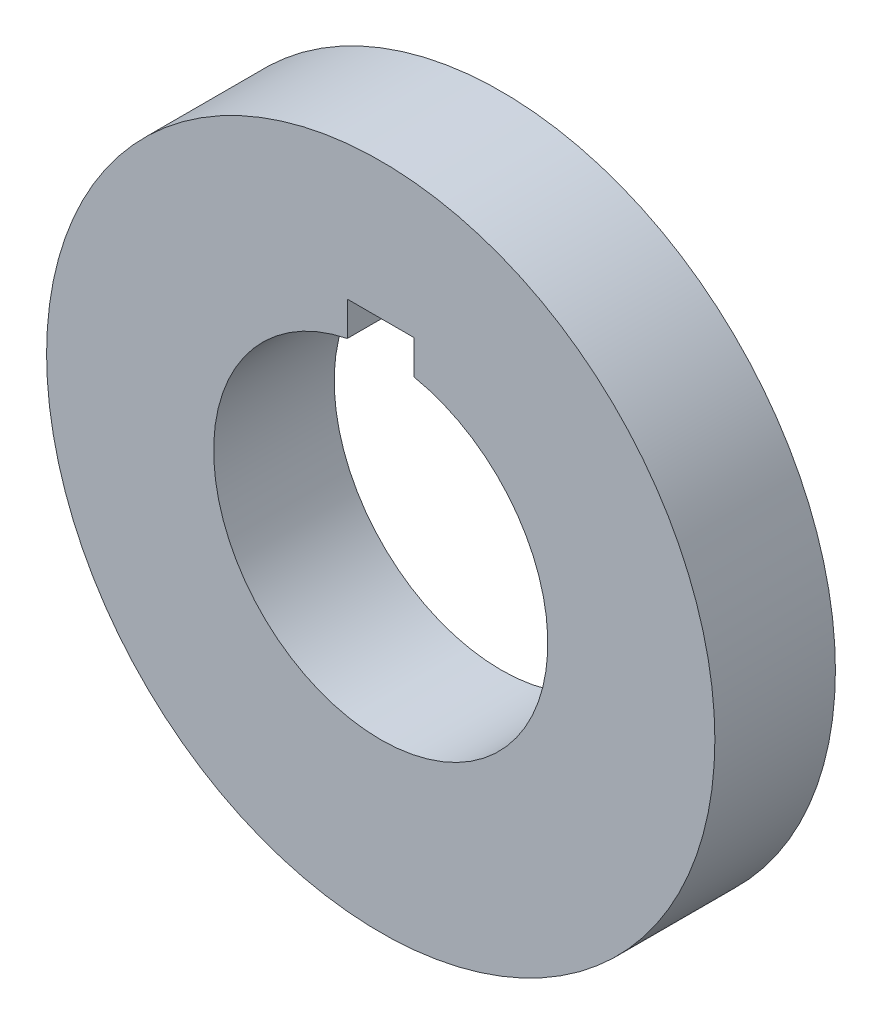
from build123d import *

# Parameters (mm, degrees)
SKETCH1_R           = 25
SKETCH1_R_2         = 12.5
BOSS_EXTRUDE1_DEPTH = 17
MOVE_FACE1_BY       = 7.981500203
SKETCH2_W           = 5
SKETCH2_H           = 4.6
CUT_EXTRUDE1_DEPTH  = 37.487440834


with BuildPart() as part:
    # Sketch1 → Boss-Extrude1 (new body)
    with BuildSketch(Plane.XY):
        Circle(SKETCH1_R)
        Circle(SKETCH1_R_2, mode=Mode.SUBTRACT)
    extrude(amount=-BOSS_EXTRUDE1_DEPTH)

    # Move Face1: a face moved inward by 7.9815
    extrude(part.faces().sort_by_distance((0, -20, 0))[0], amount=MOVE_FACE1_BY, dir=(0, 0, -1), mode=Mode.SUBTRACT)

    # Sketch2 → Cut-Extrude1 (cut, through all)
    with BuildSketch(Plane(origin=(0, 0, -17), x_dir=(-1, 0, 0), z_dir=(0, 0, -1))):
        with Locations((0, 12.5)):
            Rectangle(SKETCH2_W, SKETCH2_H)
    extrude(amount=-CUT_EXTRUDE1_DEPTH, mode=Mode.SUBTRACT)


solid = part.part
